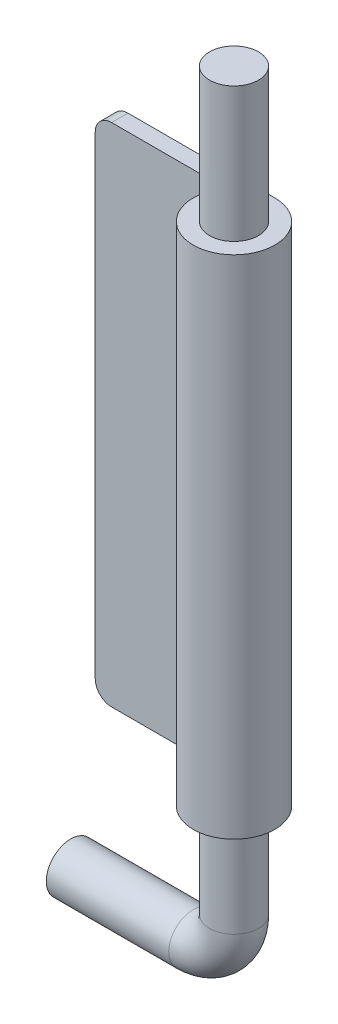
from build123d import *

# Parameters (mm, degrees)
BOSS_EXTRUDE1_DEPTH = 62
SWEEP1_PROFILE_R    = 3
FILLET3_R           = 2


with BuildPart() as part:
    # Sketch1 → Boss-Extrude1 (new body)
    with BuildSketch(Plane(origin=(0, 0, 0), x_dir=(1, 0, 0), z_dir=(0, 1, 0))):
        with BuildLine():
            Line((0, 5), (-20, 5))
            Line((-20, 5), (-20, 3))
            Line((-20, 3), (0, 3))
            ThreePointArc((0, 3), (1.826284287, -2.380060021), (-2.897777479, 0.776457135))
            Line((-2.897777479, 0.776457135), (-4.829629131, 1.294095226))
            ThreePointArc((-4.829629131, 1.294095226), (3.043807145, -3.966766701), (0, 5))
        make_face()
    extrude(amount=BOSS_EXTRUDE1_DEPTH)

    # Sweep1: sweep along a path in Sketch2
    with BuildLine(Plane.XY) as sweep1_path:
        Line((0, 78.5), (0, 0))
        Line((0, 0), (0, -11.5))
        ThreePointArc((0, -11.5), (-1.464466094, -15.035533906), (-5, -16.5))
        Line((-5, -16.5), (-20, -16.5))
    # Sweep1 profile (on start of the path) → Sweep1 (sweep)
    with BuildSketch(Plane(origin=(0, 78.5, 0), x_dir=(0, 0, -1), z_dir=(0, -1, 0))):
        Circle(SWEEP1_PROFILE_R)
    sweep(path=sweep1_path.line)

    # Fillet3
    fillet3_edges = [part.edges().sort_by_distance(p)[0] for p in [
        (-20, 62, -4),
        (-20, 0, -4),
    ]]
    fillet(fillet3_edges, radius=FILLET3_R)


solid = part.part
